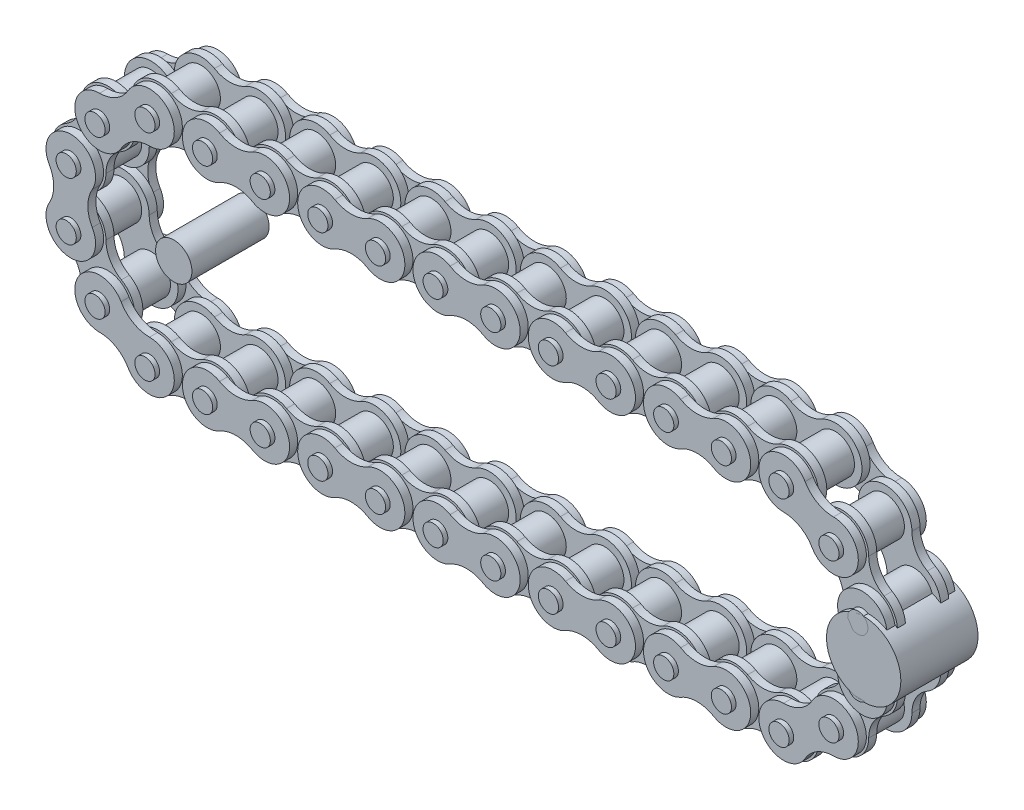
from build123d import *

# Parameters (mm, degrees)
EXTRUDE_1_DEPTH         = 8.500000462
EXTRUDE_1_DEPTH_BACK    = 8.500000462
SKETCH_1_R              = 2.224999946
EXTRUDE_1_2_DEPTH       = 8.500000462
EXTRUDE_1_2_DEPTH_BACK  = 8.500000462
EXTRUDE_1_3_DEPTH       = 8.500000462
EXTRUDE_1_3_DEPTH_BACK  = 8.500000462
EXTRUDE_1_4_DEPTH       = 8.500000462
EXTRUDE_1_4_DEPTH_BACK  = 8.500000462
EXTRUDE_1_5_DEPTH       = 8.500000462
EXTRUDE_1_5_DEPTH_BACK  = 8.500000462
EXTRUDE_1_6_DEPTH       = 8.500000462
EXTRUDE_1_6_DEPTH_BACK  = 8.500000462
EXTRUDE_1_7_DEPTH       = 8.500000462
EXTRUDE_1_7_DEPTH_BACK  = 8.500000462
EXTRUDE_1_8_DEPTH       = 8.500000462
EXTRUDE_1_8_DEPTH_BACK  = 8.500000462
EXTRUDE_1_9_DEPTH       = 8.500000462
EXTRUDE_1_9_DEPTH_BACK  = 8.500000462
EXTRUDE_1_10_DEPTH      = 8.500000462
EXTRUDE_1_10_DEPTH_BACK = 8.500000462
EXTRUDE_1_11_DEPTH      = 8.500000462
EXTRUDE_1_11_DEPTH_BACK = 8.500000462
EXTRUDE_1_12_DEPTH      = 8.500000462
EXTRUDE_1_12_DEPTH_BACK = 8.500000462
EXTRUDE_1_13_DEPTH      = 8.500000462
EXTRUDE_1_13_DEPTH_BACK = 8.500000462
EXTRUDE_1_14_DEPTH      = 8.500000462
EXTRUDE_1_14_DEPTH_BACK = 8.500000462
EXTRUDE_1_15_DEPTH      = 8.500000462
EXTRUDE_1_15_DEPTH_BACK = 8.500000462
EXTRUDE_1_16_DEPTH      = 8.500000462
EXTRUDE_1_16_DEPTH_BACK = 8.500000462
EXTRUDE_1_17_DEPTH      = 8.500000462
EXTRUDE_1_17_DEPTH_BACK = 8.500000462
EXTRUDE_1_18_DEPTH      = 8.500000462
EXTRUDE_1_18_DEPTH_BACK = 8.500000462
EXTRUDE_1_19_DEPTH      = 8.500000462
EXTRUDE_1_19_DEPTH_BACK = 8.500000462
EXTRUDE_1_20_DEPTH      = 8.500000462
EXTRUDE_1_20_DEPTH_BACK = 8.500000462
EXTRUDE_1_21_DEPTH      = 8.500000462
EXTRUDE_1_21_DEPTH_BACK = 8.500000462
EXTRUDE_1_22_DEPTH      = 8.500000462
EXTRUDE_1_22_DEPTH_BACK = 8.500000462
EXTRUDE_1_23_DEPTH      = 8.500000462
EXTRUDE_1_23_DEPTH_BACK = 8.500000462
EXTRUDE_1_24_DEPTH      = 8.500000462
EXTRUDE_1_24_DEPTH_BACK = 8.500000462
EXTRUDE_1_25_DEPTH      = 8.500000462
EXTRUDE_1_25_DEPTH_BACK = 8.500000462
EXTRUDE_1_26_DEPTH      = 8.500000462
EXTRUDE_1_26_DEPTH_BACK = 8.500000462
EXTRUDE_1_27_DEPTH      = 8.500000462
EXTRUDE_1_27_DEPTH_BACK = 8.500000462
EXTRUDE_1_28_DEPTH      = 8.500000462
EXTRUDE_1_28_DEPTH_BACK = 8.500000462
EXTRUDE_1_29_DEPTH      = 8.500000462
EXTRUDE_1_29_DEPTH_BACK = 8.500000462
EXTRUDE_1_30_DEPTH      = 8.500000462
EXTRUDE_1_30_DEPTH_BACK = 8.500000462
EXTRUDE_1_31_DEPTH      = 8.500000462
EXTRUDE_1_31_DEPTH_BACK = 8.500000462
EXTRUDE_1_32_DEPTH      = 8.500000462
EXTRUDE_1_32_DEPTH_BACK = 8.500000462
EXTRUDE_2_DEPTH         = 3.874999937
EXTRUDE_2_DEPTH_BACK    = 3.874999937
SKETCH_2_R              = 4.255000036
SKETCH_3_R              = 5.905000027
EXTRUDE_3_DEPTH         = 1.775000244
EXTRUDE_4_DEPTH         = 1.775000244
EXTRUDE_START           = 1.840000041
SKETCH_5_R              = 5.460000131
EXTRUDE_5_DEPTH         = 1.775000244
EXTRUDE_6_DEPTH         = 1.775000244
SKETCH_7_R              = 4.006025973
EXTRUDE_7_DEPTH         = 17.000000924
SKETCH_7_R_2            = 8.189187755
EXTRUDE_7_2_DEPTH       = 17.000000924


with BuildPart() as part:
    # 草图1 → 凸台-拉伸1 (new, two sides: drawn at the far end of the back side and taken through both)
    with BuildSketch(Plane.XY.offset(-EXTRUDE_1_DEPTH_BACK)):
        with Locations((-23.698522342, 6.349999923)):
            Circle(SKETCH_1_R)
    extrude(amount=EXTRUDE_1_DEPTH + EXTRUDE_1_DEPTH_BACK)



with BuildPart() as body_2:
    # 草图1 → Extrude 1 2 (new, two sides: drawn at the far end of the back side and taken through both)
    with BuildSketch(Plane.XY.offset(-EXTRUDE_1_2_DEPTH_BACK)):
        with Locations((-23.698522342, -6.349999923)):
            Circle(SKETCH_1_R)
    extrude(amount=EXTRUDE_1_2_DEPTH + EXTRUDE_1_2_DEPTH_BACK)


with BuildPart() as body_3:
    # 草图1 → Extrude 1 3 (new, two sides: drawn at the far end of the back side and taken through both)
    with BuildSketch(Plane.XY.offset(-EXTRUDE_1_3_DEPTH_BACK)):
        with Locations((150.698520807, 6.349999923)):
            Circle(SKETCH_1_R)
    extrude(amount=EXTRUDE_1_3_DEPTH + EXTRUDE_1_3_DEPTH_BACK)


with BuildPart() as body_4:
    # 草图1 → Extrude 1 4 (new, two sides: drawn at the far end of the back side and taken through both)
    with BuildSketch(Plane.XY.offset(-EXTRUDE_1_4_DEPTH_BACK)):
        with Locations((150.698520807, -6.349999923)):
            Circle(SKETCH_1_R)
    extrude(amount=EXTRUDE_1_4_DEPTH + EXTRUDE_1_4_DEPTH_BACK)


with BuildPart() as body_5:
    # 草图1 → Extrude 1 5 (new, two sides: drawn at the far end of the back side and taken through both)
    with BuildSketch(Plane.XY.offset(-EXTRUDE_1_5_DEPTH_BACK)):
        with Locations((-17.348522418, 17.348522418)):
            Circle(SKETCH_1_R)
    extrude(amount=EXTRUDE_1_5_DEPTH + EXTRUDE_1_5_DEPTH_BACK)


with BuildPart() as body_6:
    # 草图1 → Extrude 1 6 (new, two sides: drawn at the far end of the back side and taken through both)
    with BuildSketch(Plane.XY.offset(-EXTRUDE_1_6_DEPTH_BACK)):
        with Locations((-17.348522418, -17.348522418)):
            Circle(SKETCH_1_R)
    extrude(amount=EXTRUDE_1_6_DEPTH + EXTRUDE_1_6_DEPTH_BACK)


with BuildPart() as body_7:
    # 草图1 → Extrude 1 7 (new, two sides: drawn at the far end of the back side and taken through both)
    with BuildSketch(Plane.XY.offset(-EXTRUDE_1_7_DEPTH_BACK)):
        with Locations((-6.349999923, 23.698522342)):
            Circle(SKETCH_1_R)
    extrude(amount=EXTRUDE_1_7_DEPTH + EXTRUDE_1_7_DEPTH_BACK)


with BuildPart() as body_8:
    # 草图1 → Extrude 1 8 (new, two sides: drawn at the far end of the back side and taken through both)
    with BuildSketch(Plane.XY.offset(-EXTRUDE_1_8_DEPTH_BACK)):
        with Locations((-6.349999923, -23.698522342)):
            Circle(SKETCH_1_R)
    extrude(amount=EXTRUDE_1_8_DEPTH + EXTRUDE_1_8_DEPTH_BACK)


with BuildPart() as body_9:
    # 草图1 → Extrude 1 9 (new, two sides: drawn at the far end of the back side and taken through both)
    with BuildSketch(Plane.XY.offset(-EXTRUDE_1_9_DEPTH_BACK)):
        with Locations((144.348520884, 17.348522418)):
            Circle(SKETCH_1_R)
    extrude(amount=EXTRUDE_1_9_DEPTH + EXTRUDE_1_9_DEPTH_BACK)


with BuildPart() as body_10:
    # 草图1 → Extrude 1 10 (new, two sides: drawn at the far end of the back side and taken through both)
    with BuildSketch(Plane.XY.offset(-EXTRUDE_1_10_DEPTH_BACK)):
        with Locations((144.348520884, -17.348522418)):
            Circle(SKETCH_1_R)
    extrude(amount=EXTRUDE_1_10_DEPTH + EXTRUDE_1_10_DEPTH_BACK)


with BuildPart() as body_11:
    # 草图1 → Extrude 1 11 (new, two sides: drawn at the far end of the back side and taken through both)
    with BuildSketch(Plane.XY.offset(-EXTRUDE_1_11_DEPTH_BACK)):
        with Locations((133.349998388, 23.698522342)):
            Circle(SKETCH_1_R)
    extrude(amount=EXTRUDE_1_11_DEPTH + EXTRUDE_1_11_DEPTH_BACK)


with BuildPart() as body_12:
    # 草图1 → Extrude 1 12 (new, two sides: drawn at the far end of the back side and taken through both)
    with BuildSketch(Plane.XY.offset(-EXTRUDE_1_12_DEPTH_BACK)):
        with Locations((133.349998388, -23.698522342)):
            Circle(SKETCH_1_R)
    extrude(amount=EXTRUDE_1_12_DEPTH + EXTRUDE_1_12_DEPTH_BACK)


with BuildPart() as body_13:
    # 草图1 → Extrude 1 13 (new, two sides: drawn at the far end of the back side and taken through both)
    with BuildSketch(Plane.XY.offset(-EXTRUDE_1_13_DEPTH_BACK)):
        with Locations((6.349999923, 23.698522342)):
            Circle(SKETCH_1_R)
    extrude(amount=EXTRUDE_1_13_DEPTH + EXTRUDE_1_13_DEPTH_BACK)


with BuildPart() as body_14:
    # 草图1 → Extrude 1 14 (new, two sides: drawn at the far end of the back side and taken through both)
    with BuildSketch(Plane.XY.offset(-EXTRUDE_1_14_DEPTH_BACK)):
        with Locations((6.349999923, -23.698522342)):
            Circle(SKETCH_1_R)
    extrude(amount=EXTRUDE_1_14_DEPTH + EXTRUDE_1_14_DEPTH_BACK)


with BuildPart() as body_15:
    # 草图1 → Extrude 1 15 (new, two sides: drawn at the far end of the back side and taken through both)
    with BuildSketch(Plane.XY.offset(-EXTRUDE_1_15_DEPTH_BACK)):
        with Locations((19.04999977, 23.698522342)):
            Circle(SKETCH_1_R)
    extrude(amount=EXTRUDE_1_15_DEPTH + EXTRUDE_1_15_DEPTH_BACK)


with BuildPart() as body_16:
    # 草图1 → Extrude 1 16 (new, two sides: drawn at the far end of the back side and taken through both)
    with BuildSketch(Plane.XY.offset(-EXTRUDE_1_16_DEPTH_BACK)):
        with Locations((19.04999977, -23.698522342)):
            Circle(SKETCH_1_R)
    extrude(amount=EXTRUDE_1_16_DEPTH + EXTRUDE_1_16_DEPTH_BACK)


with BuildPart() as body_17:
    # 草图1 → Extrude 1 17 (new, two sides: drawn at the far end of the back side and taken through both)
    with BuildSketch(Plane.XY.offset(-EXTRUDE_1_17_DEPTH_BACK)):
        with Locations((31.749999616, 23.698522342)):
            Circle(SKETCH_1_R)
    extrude(amount=EXTRUDE_1_17_DEPTH + EXTRUDE_1_17_DEPTH_BACK)


with BuildPart() as body_18:
    # 草图1 → Extrude 1 18 (new, two sides: drawn at the far end of the back side and taken through both)
    with BuildSketch(Plane.XY.offset(-EXTRUDE_1_18_DEPTH_BACK)):
        with Locations((31.749999616, -23.698522342)):
            Circle(SKETCH_1_R)
    extrude(amount=EXTRUDE_1_18_DEPTH + EXTRUDE_1_18_DEPTH_BACK)


with BuildPart() as body_19:
    # 草图1 → Extrude 1 19 (new, two sides: drawn at the far end of the back side and taken through both)
    with BuildSketch(Plane.XY.offset(-EXTRUDE_1_19_DEPTH_BACK)):
        with Locations((44.449999463, 23.698522342)):
            Circle(SKETCH_1_R)
    extrude(amount=EXTRUDE_1_19_DEPTH + EXTRUDE_1_19_DEPTH_BACK)


with BuildPart() as body_20:
    # 草图1 → Extrude 1 20 (new, two sides: drawn at the far end of the back side and taken through both)
    with BuildSketch(Plane.XY.offset(-EXTRUDE_1_20_DEPTH_BACK)):
        with Locations((44.449999463, -23.698522342)):
            Circle(SKETCH_1_R)
    extrude(amount=EXTRUDE_1_20_DEPTH + EXTRUDE_1_20_DEPTH_BACK)


with BuildPart() as body_21:
    # 草图1 → Extrude 1 21 (new, two sides: drawn at the far end of the back side and taken through both)
    with BuildSketch(Plane.XY.offset(-EXTRUDE_1_21_DEPTH_BACK)):
        with Locations((57.149999309, 23.698522342)):
            Circle(SKETCH_1_R)
    extrude(amount=EXTRUDE_1_21_DEPTH + EXTRUDE_1_21_DEPTH_BACK)


with BuildPart() as body_22:
    # 草图1 → Extrude 1 22 (new, two sides: drawn at the far end of the back side and taken through both)
    with BuildSketch(Plane.XY.offset(-EXTRUDE_1_22_DEPTH_BACK)):
        with Locations((57.149999309, -23.698522342)):
            Circle(SKETCH_1_R)
    extrude(amount=EXTRUDE_1_22_DEPTH + EXTRUDE_1_22_DEPTH_BACK)


with BuildPart() as body_23:
    # 草图1 → Extrude 1 23 (new, two sides: drawn at the far end of the back side and taken through both)
    with BuildSketch(Plane.XY.offset(-EXTRUDE_1_23_DEPTH_BACK)):
        with Locations((69.849999156, 23.698522342)):
            Circle(SKETCH_1_R)
    extrude(amount=EXTRUDE_1_23_DEPTH + EXTRUDE_1_23_DEPTH_BACK)


with BuildPart() as body_24:
    # 草图1 → Extrude 1 24 (new, two sides: drawn at the far end of the back side and taken through both)
    with BuildSketch(Plane.XY.offset(-EXTRUDE_1_24_DEPTH_BACK)):
        with Locations((69.849999156, -23.698522342)):
            Circle(SKETCH_1_R)
    extrude(amount=EXTRUDE_1_24_DEPTH + EXTRUDE_1_24_DEPTH_BACK)


with BuildPart() as body_25:
    # 草图1 → Extrude 1 25 (new, two sides: drawn at the far end of the back side and taken through both)
    with BuildSketch(Plane.XY.offset(-EXTRUDE_1_25_DEPTH_BACK)):
        with Locations((82.549999002, 23.698522342)):
            Circle(SKETCH_1_R)
    extrude(amount=EXTRUDE_1_25_DEPTH + EXTRUDE_1_25_DEPTH_BACK)


with BuildPart() as body_26:
    # 草图1 → Extrude 1 26 (new, two sides: drawn at the far end of the back side and taken through both)
    with BuildSketch(Plane.XY.offset(-EXTRUDE_1_26_DEPTH_BACK)):
        with Locations((82.549999002, -23.698522342)):
            Circle(SKETCH_1_R)
    extrude(amount=EXTRUDE_1_26_DEPTH + EXTRUDE_1_26_DEPTH_BACK)


with BuildPart() as body_27:
    # 草图1 → Extrude 1 27 (new, two sides: drawn at the far end of the back side and taken through both)
    with BuildSketch(Plane.XY.offset(-EXTRUDE_1_27_DEPTH_BACK)):
        with Locations((95.249998849, 23.698522342)):
            Circle(SKETCH_1_R)
    extrude(amount=EXTRUDE_1_27_DEPTH + EXTRUDE_1_27_DEPTH_BACK)


with BuildPart() as body_28:
    # 草图1 → Extrude 1 28 (new, two sides: drawn at the far end of the back side and taken through both)
    with BuildSketch(Plane.XY.offset(-EXTRUDE_1_28_DEPTH_BACK)):
        with Locations((95.249998849, -23.698522342)):
            Circle(SKETCH_1_R)
    extrude(amount=EXTRUDE_1_28_DEPTH + EXTRUDE_1_28_DEPTH_BACK)


with BuildPart() as body_29:
    # 草图1 → Extrude 1 29 (new, two sides: drawn at the far end of the back side and taken through both)
    with BuildSketch(Plane.XY.offset(-EXTRUDE_1_29_DEPTH_BACK)):
        with Locations((107.949998695, 23.698522342)):
            Circle(SKETCH_1_R)
    extrude(amount=EXTRUDE_1_29_DEPTH + EXTRUDE_1_29_DEPTH_BACK)


with BuildPart() as body_30:
    # 草图1 → Extrude 1 30 (new, two sides: drawn at the far end of the back side and taken through both)
    with BuildSketch(Plane.XY.offset(-EXTRUDE_1_30_DEPTH_BACK)):
        with Locations((107.949998695, -23.698522342)):
            Circle(SKETCH_1_R)
    extrude(amount=EXTRUDE_1_30_DEPTH + EXTRUDE_1_30_DEPTH_BACK)


with BuildPart() as body_31:
    # 草图1 → Extrude 1 31 (new, two sides: drawn at the far end of the back side and taken through both)
    with BuildSketch(Plane.XY.offset(-EXTRUDE_1_31_DEPTH_BACK)):
        with Locations((120.649998542, 23.698522342)):
            Circle(SKETCH_1_R)
    extrude(amount=EXTRUDE_1_31_DEPTH + EXTRUDE_1_31_DEPTH_BACK)


with BuildPart() as body_32:
    # 草图1 → Extrude 1 32 (new, two sides: drawn at the far end of the back side and taken through both)
    with BuildSketch(Plane.XY.offset(-EXTRUDE_1_32_DEPTH_BACK)):
        with Locations((120.649998542, -23.698522342)):
            Circle(SKETCH_1_R)
    extrude(amount=EXTRUDE_1_32_DEPTH + EXTRUDE_1_32_DEPTH_BACK)


with BuildPart() as part_1:
    add(part.part)

    add(body_2.part)  # 凸台-拉伸2 merges body 2

    add(body_3.part)  # 凸台-拉伸2 merges body 3

    add(body_4.part)  # 凸台-拉伸2 merges body 4

    add(body_5.part)  # 凸台-拉伸2 merges body 5

    add(body_6.part)  # 凸台-拉伸2 merges body 6

    add(body_7.part)  # 凸台-拉伸2 merges body 7

    add(body_8.part)  # 凸台-拉伸2 merges body 8

    add(body_9.part)  # 凸台-拉伸2 merges body 9

    add(body_10.part)  # 凸台-拉伸2 merges body 10

    add(body_11.part)  # 凸台-拉伸2 merges body 11

    add(body_12.part)  # 凸台-拉伸2 merges body 12

    add(body_13.part)  # 凸台-拉伸2 merges body 13

    add(body_14.part)  # 凸台-拉伸2 merges body 14

    add(body_15.part)  # 凸台-拉伸2 merges body 15

    add(body_16.part)  # 凸台-拉伸2 merges body 16

    add(body_17.part)  # 凸台-拉伸2 merges body 17

    add(body_18.part)  # 凸台-拉伸2 merges body 18

    add(body_19.part)  # 凸台-拉伸2 merges body 19

    add(body_20.part)  # 凸台-拉伸2 merges body 20

    add(body_21.part)  # 凸台-拉伸2 merges body 21

    add(body_22.part)  # 凸台-拉伸2 merges body 22

    add(body_23.part)  # 凸台-拉伸2 merges body 23

    add(body_24.part)  # 凸台-拉伸2 merges body 24

    add(body_25.part)  # 凸台-拉伸2 merges body 25

    add(body_26.part)  # 凸台-拉伸2 merges body 26

    add(body_27.part)  # 凸台-拉伸2 merges body 27

    add(body_28.part)  # 凸台-拉伸2 merges body 28

    add(body_29.part)  # 凸台-拉伸2 merges body 29

    add(body_30.part)  # 凸台-拉伸2 merges body 30

    add(body_31.part)  # 凸台-拉伸2 merges body 31

    add(body_32.part)  # 凸台-拉伸2 merges body 32
    # 草图2 → 凸台-拉伸2 (add, two sides: drawn at the far end of the back side and taken through both)
    with BuildSketch(Plane.XY.offset(-EXTRUDE_2_DEPTH_BACK)):
        with Locations((-23.698522342, 6.349999923)):
            Circle(SKETCH_2_R)
        with Locations((-23.698522342, -6.349999923)):
            Circle(SKETCH_2_R)
        with Locations((150.698520807, 6.349999923)):
            Circle(SKETCH_2_R)
        with Locations((150.698520807, -6.349999923)):
            Circle(SKETCH_2_R)
        with Locations((-17.348522418, 17.348522418)):
            Circle(SKETCH_2_R)
        with Locations((-17.348522418, -17.348522418)):
            Circle(SKETCH_2_R)
        with Locations((-6.349999923, 23.698522342)):
            Circle(SKETCH_2_R)
        with Locations((-6.349999923, -23.698522342)):
            Circle(SKETCH_2_R)
        with Locations((144.348520884, 17.348522418)):
            Circle(SKETCH_2_R)
        with Locations((144.348520884, -17.348522418)):
            Circle(SKETCH_2_R)
        with Locations((133.349998388, 23.698522342)):
            Circle(SKETCH_2_R)
        with Locations((133.349998388, -23.698522342)):
            Circle(SKETCH_2_R)
        with Locations((6.349999923, 23.698522342)):
            Circle(SKETCH_2_R)
        with Locations((6.349999923, -23.698522342)):
            Circle(SKETCH_2_R)
        with Locations((19.04999977, 23.698522342)):
            Circle(SKETCH_2_R)
        with Locations((19.04999977, -23.698522342)):
            Circle(SKETCH_2_R)
        with Locations((31.749999616, 23.698522342)):
            Circle(SKETCH_2_R)
        with Locations((31.749999616, -23.698522342)):
            Circle(SKETCH_2_R)
        with Locations((44.449999463, 23.698522342)):
            Circle(SKETCH_2_R)
        with Locations((44.449999463, -23.698522342)):
            Circle(SKETCH_2_R)
        with Locations((57.149999309, 23.698522342)):
            Circle(SKETCH_2_R)
        with Locations((57.149999309, -23.698522342)):
            Circle(SKETCH_2_R)
        with Locations((69.849999156, 23.698522342)):
            Circle(SKETCH_2_R)
        with Locations((69.849999156, -23.698522342)):
            Circle(SKETCH_2_R)
        with Locations((82.549999002, 23.698522342)):
            Circle(SKETCH_2_R)
        with Locations((82.549999002, -23.698522342)):
            Circle(SKETCH_2_R)
        with Locations((95.249998849, 23.698522342)):
            Circle(SKETCH_2_R)
        with Locations((95.249998849, -23.698522342)):
            Circle(SKETCH_2_R)
        with Locations((107.949998695, 23.698522342)):
            Circle(SKETCH_2_R)
        with Locations((107.949998695, -23.698522342)):
            Circle(SKETCH_2_R)
        with Locations((120.649998542, 23.698522342)):
            Circle(SKETCH_2_R)
        with Locations((120.649998542, -23.698522342)):
            Circle(SKETCH_2_R)
    extrude(amount=EXTRUDE_2_DEPTH + EXTRUDE_2_DEPTH_BACK)

    # 草图3 → 凸台-拉伸3 (add)
    with BuildSketch(Plane.XY.offset(3.874999937)):
        with Locations(Location((-23.698522342, 6.349999923, 0), (0, 0, 180))):
            Circle(SKETCH_3_R)
        with Locations(Location((-23.698522342, -6.349999923, 0), (0, 0, 180))):
            Circle(SKETCH_3_R)
        with Locations(Location((150.698520807, 6.349999923, 0), (0, 0, 180))):
            Circle(SKETCH_3_R)
        with Locations(Location((150.698520807, -6.349999923, 0), (0, 0, 180))):
            Circle(SKETCH_3_R)
        with Locations(Location((-17.348522418, 17.348522418, 0), (0, 0, 180))):
            Circle(SKETCH_3_R)
        with Locations(Location((-17.348522418, -17.348522418, 0), (0, 0, 180))):
            Circle(SKETCH_3_R)
        with Locations(Location((-6.349999923, 23.698522342, 0), (0, 0, 180))):
            Circle(SKETCH_3_R)
        with Locations(Location((-6.349999923, -23.698522342, 0), (0, 0, 180))):
            Circle(SKETCH_3_R)
        with Locations(Location((144.348520884, 17.348522418, 0), (0, 0, 180))):
            Circle(SKETCH_3_R)
        with Locations(Location((144.348520884, -17.348522418, 0), (0, 0, 180))):
            Circle(SKETCH_3_R)
        with Locations(Location((133.349998388, 23.698522342, 0), (0, 0, 180))):
            Circle(SKETCH_3_R)
        with Locations(Location((133.349998388, -23.698522342, 0), (0, 0, 180))):
            Circle(SKETCH_3_R)
        with Locations(Location((6.349999923, 23.698522342, 0), (0, 0, 180))):
            Circle(SKETCH_3_R)
        with Locations(Location((6.349999923, -23.698522342, 0), (0, 0, 180))):
            Circle(SKETCH_3_R)
        with Locations(Location((19.04999977, 23.698522342, 0), (0, 0, 180))):
            Circle(SKETCH_3_R)
        with Locations(Location((19.04999977, -23.698522342, 0), (0, 0, 180))):
            Circle(SKETCH_3_R)
        with Locations(Location((31.749999616, 23.698522342, 0), (0, 0, 180))):
            Circle(SKETCH_3_R)
        with Locations(Location((31.749999616, -23.698522342, 0), (0, 0, 180))):
            Circle(SKETCH_3_R)
        with Locations(Location((44.449999463, 23.698522342, 0), (0, 0, 180))):
            Circle(SKETCH_3_R)
        with Locations(Location((44.449999463, -23.698522342, 0), (0, 0, 180))):
            Circle(SKETCH_3_R)
        with Locations(Location((57.149999309, 23.698522342, 0), (0, 0, 180))):
            Circle(SKETCH_3_R)
        with Locations(Location((57.149999309, -23.698522342, 0), (0, 0, 180))):
            Circle(SKETCH_3_R)
        with Locations(Location((69.849999156, 23.698522342, 0), (0, 0, 180))):
            Circle(SKETCH_3_R)
        with Locations(Location((69.849999156, -23.698522342, 0), (0, 0, 180))):
            Circle(SKETCH_3_R)
        with Locations(Location((82.549999002, 23.698522342, 0), (0, 0, 180))):
            Circle(SKETCH_3_R)
        with Locations(Location((82.549999002, -23.698522342, 0), (0, 0, 180))):
            Circle(SKETCH_3_R)
        with Locations(Location((95.249998849, 23.698522342, 0), (0, 0, 180))):
            Circle(SKETCH_3_R)
        with Locations(Location((95.249998849, -23.698522342, 0), (0, 0, 180))):
            Circle(SKETCH_3_R)
        with Locations(Location((107.949998695, 23.698522342, 0), (0, 0, 180))):
            Circle(SKETCH_3_R)
        with Locations(Location((107.949998695, -23.698522342, 0), (0, 0, 180))):
            Circle(SKETCH_3_R)
        with Locations(Location((120.649998542, 23.698522342, 0), (0, 0, 180))):
            Circle(SKETCH_3_R)
        with Locations(Location((120.649998542, -23.698522342, 0), (0, 0, 180))):
            Circle(SKETCH_3_R)
    extrude_3 = extrude(amount=EXTRUDE_3_DEPTH)

    # 草图4 → 凸台-拉伸4 (add)
    with BuildSketch(Plane.XY.offset(3.874999937)):
        with BuildLine():
            Line((-26.651022364, 11.463879961), (-17.793522323, 6.349999928))
            ThreePointArc((-17.793522323, 6.349999928), (-16.883164966, 9.747499838), (-14.396022414, 12.234642391))
            Line((-14.396022414, 12.234642391), (-23.253522455, 17.348522424))
            ThreePointArc((-23.253522455, 17.348522424), (-24.163879812, 13.951022514), (-26.651022364, 11.463879961))
        make_face()
        with BuildLine():
            Line((-26.651022364, -11.463879961), (-17.793522323, -6.349999928))
            ThreePointArc((-17.793522323, -6.349999928), (-16.883164966, -9.747499838), (-14.396022414, -12.234642391))
            Line((-14.396022414, -12.234642391), (-23.253522455, -17.348522424))
            ThreePointArc((-23.253522455, -17.348522424), (-24.163879812, -13.951022514), (-26.651022364, -11.463879961))
        make_face()
        with BuildLine():
            Line((153.65102082, 11.463879956), (144.79352078, 6.349999923))
            ThreePointArc((144.79352078, 6.349999923), (143.883163423, 9.747499833), (141.39602087, 12.234642385))
            Line((141.39602087, 12.234642385), (150.253520911, 17.348522418))
            ThreePointArc((150.253520911, 17.348522418), (151.163878268, 13.951022509), (153.65102082, 11.463879956))
        make_face()
        with BuildLine():
            Line((153.65102082, -11.463879956), (144.79352078, -6.349999923))
            ThreePointArc((144.79352078, -6.349999923), (143.883163423, -9.747499833), (141.39602087, -12.234642385))
            Line((141.39602087, -12.234642385), (150.253520911, -17.348522418))
            ThreePointArc((150.253520911, -17.348522418), (151.163878268, -13.951022509), (153.65102082, -11.463879956))
        make_face()
        with BuildLine():
            Line((-3.39749991, 28.812402375), (-3.39749991, 18.584642309))
            ThreePointArc((-3.39749991, 18.584642309), (0, 19.494999666), (3.39749991, 18.584642309))
            Line((3.39749991, 18.584642309), (3.39749991, 28.812402375))
            ThreePointArc((3.39749991, 28.812402375), (0, 27.902045018), (-3.39749991, 28.812402375))
        make_face()
        with BuildLine():
            Line((-3.39749991, -28.812402375), (-3.39749991, -18.584642309))
            ThreePointArc((-3.39749991, -18.584642309), (0, -19.494999666), (3.39749991, -18.584642309))
            Line((3.39749991, -18.584642309), (3.39749991, -28.812402375))
            ThreePointArc((3.39749991, -28.812402375), (0, -27.902045018), (-3.39749991, -28.812402375))
        make_face()
        with BuildLine():
            Line((22.002499783, 28.812402375), (22.002499783, 18.584642309))
            ThreePointArc((22.002499783, 18.584642309), (25.399999693, 19.494999666), (28.797499603, 18.584642309))
            Line((28.797499603, 18.584642309), (28.797499603, 28.812402375))
            ThreePointArc((28.797499603, 28.812402375), (25.399999693, 27.902045018), (22.002499783, 28.812402375))
        make_face()
        with BuildLine():
            Line((22.002499783, -28.812402375), (22.002499783, -18.584642309))
            ThreePointArc((22.002499783, -18.584642309), (25.399999693, -19.494999666), (28.797499603, -18.584642309))
            Line((28.797499603, -18.584642309), (28.797499603, -28.812402375))
            ThreePointArc((28.797499603, -28.812402375), (25.399999693, -27.902045018), (22.002499783, -28.812402375))
        make_face()
        with BuildLine():
            Line((47.402499476, 28.812402375), (47.402499476, 18.584642309))
            ThreePointArc((47.402499476, 18.584642309), (50.799999386, 19.494999666), (54.197499296, 18.584642309))
            Line((54.197499296, 18.584642309), (54.197499296, 28.812402375))
            ThreePointArc((54.197499296, 28.812402375), (50.799999386, 27.902045018), (47.402499476, 28.812402375))
        make_face()
        with BuildLine():
            Line((47.402499476, -28.812402375), (47.402499476, -18.584642309))
            ThreePointArc((47.402499476, -18.584642309), (50.799999386, -19.494999666), (54.197499296, -18.584642309))
            Line((54.197499296, -18.584642309), (54.197499296, -28.812402375))
            ThreePointArc((54.197499296, -28.812402375), (50.799999386, -27.902045018), (47.402499476, -28.812402375))
        make_face()
        with BuildLine():
            Line((72.802499169, 28.812402375), (72.802499169, 18.584642309))
            ThreePointArc((72.802499169, 18.584642309), (76.199999079, 19.494999666), (79.597498989, 18.584642309))
            Line((79.597498989, 18.584642309), (79.597498989, 28.812402375))
            ThreePointArc((79.597498989, 28.812402375), (76.199999079, 27.902045018), (72.802499169, 28.812402375))
        make_face()
        with BuildLine():
            Line((72.802499169, -28.812402375), (72.802499169, -18.584642309))
            ThreePointArc((72.802499169, -18.584642309), (76.199999079, -19.494999666), (79.597498989, -18.584642309))
            Line((79.597498989, -18.584642309), (79.597498989, -28.812402375))
            ThreePointArc((79.597498989, -28.812402375), (76.199999079, -27.902045018), (72.802499169, -28.812402375))
        make_face()
        with BuildLine():
            Line((98.202498863, 28.812402375), (98.202498863, 18.584642309))
            ThreePointArc((98.202498863, 18.584642309), (101.599998772, 19.494999666), (104.997498682, 18.584642309))
            Line((104.997498682, 18.584642309), (104.997498682, 28.812402375))
            ThreePointArc((104.997498682, 28.812402375), (101.599998772, 27.902045018), (98.202498863, 28.812402375))
        make_face()
        with BuildLine():
            Line((98.202498863, -28.812402375), (98.202498863, -18.584642309))
            ThreePointArc((98.202498863, -18.584642309), (101.599998772, -19.494999666), (104.997498682, -18.584642309))
            Line((104.997498682, -18.584642309), (104.997498682, -28.812402375))
            ThreePointArc((104.997498682, -28.812402375), (101.599998772, -27.902045018), (98.202498863, -28.812402375))
        make_face()
        with BuildLine():
            Line((123.602498556, 28.812402375), (123.602498556, 18.584642309))
            ThreePointArc((123.602498556, 18.584642309), (126.999998465, 19.494999666), (130.397498375, 18.584642309))
            Line((130.397498375, 18.584642309), (130.397498375, 28.812402375))
            ThreePointArc((130.397498375, 28.812402375), (126.999998465, 27.902045018), (123.602498556, 28.812402375))
        make_face()
        with BuildLine():
            Line((123.602498556, -28.812402375), (123.602498556, -18.584642309))
            ThreePointArc((123.602498556, -18.584642309), (126.999998465, -19.494999666), (130.397498375, -18.584642309))
            Line((130.397498375, -18.584642309), (130.397498375, -28.812402375))
            ThreePointArc((130.397498375, -28.812402375), (126.999998465, -27.902045018), (123.602498556, -28.812402375))
        make_face()
    extrude_4 = extrude(amount=EXTRUDE_4_DEPTH)

    # 草图5 → 凸台-拉伸5 (add)
    with BuildSketch(Plane.XY.offset(3.874999937).offset(EXTRUDE_START)):
        with Locations(Location((-23.698522342, 6.349999923, 0), (0, 0, 180))):
            Circle(SKETCH_5_R)
        with Locations(Location((-23.698522342, -6.349999923, 0), (0, 0, 180))):
            Circle(SKETCH_5_R)
        with Locations(Location((150.698520807, 6.349999923, 0), (0, 0, 180))):
            Circle(SKETCH_5_R)
        with Locations(Location((150.698520807, -6.349999923, 0), (0, 0, 180))):
            Circle(SKETCH_5_R)
        with Locations(Location((-17.348522418, 17.348522418, 0), (0, 0, 180))):
            Circle(SKETCH_5_R)
        with Locations(Location((-17.348522418, -17.348522418, 0), (0, 0, 180))):
            Circle(SKETCH_5_R)
        with Locations(Location((-6.349999923, 23.698522342, 0), (0, 0, 180))):
            Circle(SKETCH_5_R)
        with Locations(Location((-6.349999923, -23.698522342, 0), (0, 0, 180))):
            Circle(SKETCH_5_R)
        with Locations(Location((144.348520884, 17.348522418, 0), (0, 0, 180))):
            Circle(SKETCH_5_R)
        with Locations(Location((144.348520884, -17.348522418, 0), (0, 0, 180))):
            Circle(SKETCH_5_R)
        with Locations(Location((133.349998388, 23.698522342, 0), (0, 0, 180))):
            Circle(SKETCH_5_R)
        with Locations(Location((133.349998388, -23.698522342, 0), (0, 0, 180))):
            Circle(SKETCH_5_R)
        with Locations(Location((6.349999923, 23.698522342, 0), (0, 0, 180))):
            Circle(SKETCH_5_R)
        with Locations(Location((6.349999923, -23.698522342, 0), (0, 0, 180))):
            Circle(SKETCH_5_R)
        with Locations(Location((19.04999977, 23.698522342, 0), (0, 0, 180))):
            Circle(SKETCH_5_R)
        with Locations(Location((19.04999977, -23.698522342, 0), (0, 0, 180))):
            Circle(SKETCH_5_R)
        with Locations(Location((31.749999616, 23.698522342, 0), (0, 0, 180))):
            Circle(SKETCH_5_R)
        with Locations(Location((31.749999616, -23.698522342, 0), (0, 0, 180))):
            Circle(SKETCH_5_R)
        with Locations(Location((44.449999463, 23.698522342, 0), (0, 0, 180))):
            Circle(SKETCH_5_R)
        with Locations(Location((44.449999463, -23.698522342, 0), (0, 0, 180))):
            Circle(SKETCH_5_R)
        with Locations(Location((57.149999309, 23.698522342, 0), (0, 0, 180))):
            Circle(SKETCH_5_R)
        with Locations(Location((57.149999309, -23.698522342, 0), (0, 0, 180))):
            Circle(SKETCH_5_R)
        with Locations(Location((69.849999156, 23.698522342, 0), (0, 0, 180))):
            Circle(SKETCH_5_R)
        with Locations(Location((69.849999156, -23.698522342, 0), (0, 0, 180))):
            Circle(SKETCH_5_R)
        with Locations(Location((82.549999002, 23.698522342, 0), (0, 0, 180))):
            Circle(SKETCH_5_R)
        with Locations(Location((82.549999002, -23.698522342, 0), (0, 0, 180))):
            Circle(SKETCH_5_R)
        with Locations(Location((95.249998849, 23.698522342, 0), (0, 0, 180))):
            Circle(SKETCH_5_R)
        with Locations(Location((95.249998849, -23.698522342, 0), (0, 0, 180))):
            Circle(SKETCH_5_R)
        with Locations(Location((107.949998695, 23.698522342, 0), (0, 0, 180))):
            Circle(SKETCH_5_R)
        with Locations(Location((107.949998695, -23.698522342, 0), (0, 0, 180))):
            Circle(SKETCH_5_R)
        with Locations(Location((120.649998542, 23.698522342, 0), (0, 0, 180))):
            Circle(SKETCH_5_R)
        with Locations(Location((120.649998542, -23.698522342, 0), (0, 0, 180))):
            Circle(SKETCH_5_R)
    extrude_5 = extrude(amount=EXTRUDE_5_DEPTH)

    # 草图6 → 凸台-拉伸6 (add)
    with BuildSketch(Plane.XY.offset(3.874999937).offset(EXTRUDE_START)):
        with BuildLine():
            Line((-28.42702117, 3.619999858), (-18.970023534, 3.619999858))
            ThreePointArc((-18.970023534, 3.619999858), (-19.939999572, 0), (-18.970023534, -3.619999858))
            Line((-18.970023534, -3.619999858), (-28.42702117, -3.619999858))
            ThreePointArc((-28.42702117, -3.619999858), (-27.457045132, 0), (-28.42702117, 3.619999858))
        make_face()
        with BuildLine():
            Line((155.427019625, 3.619999858), (145.970021988, 3.619999858))
            ThreePointArc((145.970021988, 3.619999858), (146.939998027, 0), (145.970021988, -3.619999858))
            Line((145.970021988, -3.619999858), (155.427019625, -3.619999858))
            ThreePointArc((155.427019625, -3.619999858), (154.457043587, 0), (155.427019625, 3.619999858))
        make_face()
        with BuildLine():
            Line((-17.348522424, 22.808522559), (-12.620023605, 14.618522362))
            ThreePointArc((-12.620023605, 14.618522362), (-9.969999786, 17.268546181), (-6.349999928, 18.238522219))
            Line((-6.349999928, 18.238522219), (-11.078498747, 26.428522416))
            ThreePointArc((-11.078498747, 26.428522416), (-13.728522566, 23.778498597), (-17.348522424, 22.808522559))
        make_face()
        with BuildLine():
            Line((-17.348522424, -22.808522559), (-12.620023605, -14.618522362))
            ThreePointArc((-12.620023605, -14.618522362), (-9.969999786, -17.268546181), (-6.349999928, -18.238522219))
            Line((-6.349999928, -18.238522219), (-11.078498747, -26.428522416))
            ThreePointArc((-11.078498747, -26.428522416), (-13.728522566, -23.778498597), (-17.348522424, -22.808522559))
        make_face()
        with BuildLine():
            Line((144.348520884, 22.80852255), (139.620022065, 14.618522353))
            ThreePointArc((139.620022065, 14.618522353), (136.969998246, 17.268546172), (133.349998388, 18.23852221))
            Line((133.349998388, 18.23852221), (138.078497207, 26.428522407))
            ThreePointArc((138.078497207, 26.428522407), (140.728521026, 23.778498588), (144.348520884, 22.80852255))
        make_face()
        with BuildLine():
            Line((144.348520884, -22.80852255), (139.620022065, -14.618522353))
            ThreePointArc((139.620022065, -14.618522353), (136.969998246, -17.268546172), (133.349998388, -18.23852221))
            Line((133.349998388, -18.23852221), (138.078497207, -26.428522407))
            ThreePointArc((138.078497207, -26.428522407), (140.728521026, -23.778498588), (144.348520884, -22.80852255))
        make_face()
        with BuildLine():
            Line((9.079999989, 28.42702116), (9.079999989, 18.970023523))
            ThreePointArc((9.079999989, 18.970023523), (12.699999847, 19.939999562), (16.319999704, 18.970023523))
            Line((16.319999704, 18.970023523), (16.319999704, 28.42702116))
            ThreePointArc((16.319999704, 28.42702116), (12.699999847, 27.457045122), (9.079999989, 28.42702116))
        make_face()
        with BuildLine():
            Line((9.079999989, -28.42702116), (9.079999989, -18.970023523))
            ThreePointArc((9.079999989, -18.970023523), (12.699999847, -19.939999562), (16.319999704, -18.970023523))
            Line((16.319999704, -18.970023523), (16.319999704, -28.42702116))
            ThreePointArc((16.319999704, -28.42702116), (12.699999847, -27.457045122), (9.079999989, -28.42702116))
        make_face()
        with BuildLine():
            Line((34.479999682, 28.42702116), (34.479999682, 18.970023523))
            ThreePointArc((34.479999682, 18.970023523), (38.09999954, 19.939999562), (41.719999397, 18.970023523))
            Line((41.719999397, 18.970023523), (41.719999397, 28.42702116))
            ThreePointArc((41.719999397, 28.42702116), (38.09999954, 27.457045122), (34.479999682, 28.42702116))
        make_face()
        with BuildLine():
            Line((34.479999682, -28.42702116), (34.479999682, -18.970023523))
            ThreePointArc((34.479999682, -18.970023523), (38.09999954, -19.939999562), (41.719999397, -18.970023523))
            Line((41.719999397, -18.970023523), (41.719999397, -28.42702116))
            ThreePointArc((41.719999397, -28.42702116), (38.09999954, -27.457045122), (34.479999682, -28.42702116))
        make_face()
        with BuildLine():
            Line((59.879999375, 28.42702116), (59.879999375, 18.970023523))
            ThreePointArc((59.879999375, 18.970023523), (63.499999233, 19.939999562), (67.11999909, 18.970023523))
            Line((67.11999909, 18.970023523), (67.11999909, 28.42702116))
            ThreePointArc((67.11999909, 28.42702116), (63.499999233, 27.457045122), (59.879999375, 28.42702116))
        make_face()
        with BuildLine():
            Line((59.879999375, -28.42702116), (59.879999375, -18.970023523))
            ThreePointArc((59.879999375, -18.970023523), (63.499999233, -19.939999562), (67.11999909, -18.970023523))
            Line((67.11999909, -18.970023523), (67.11999909, -28.42702116))
            ThreePointArc((67.11999909, -28.42702116), (63.499999233, -27.457045122), (59.879999375, -28.42702116))
        make_face()
        with BuildLine():
            Line((85.279999068, 28.42702116), (85.279999068, 18.970023523))
            ThreePointArc((85.279999068, 18.970023523), (88.899998926, 19.939999562), (92.519998783, 18.970023523))
            Line((92.519998783, 18.970023523), (92.519998783, 28.42702116))
            ThreePointArc((92.519998783, 28.42702116), (88.899998926, 27.457045122), (85.279999068, 28.42702116))
        make_face()
        with BuildLine():
            Line((85.279999068, -28.42702116), (85.279999068, -18.970023523))
            ThreePointArc((85.279999068, -18.970023523), (88.899998926, -19.939999562), (92.519998783, -18.970023523))
            Line((92.519998783, -18.970023523), (92.519998783, -28.42702116))
            ThreePointArc((92.519998783, -28.42702116), (88.899998926, -27.457045122), (85.279999068, -28.42702116))
        make_face()
        with BuildLine():
            Line((110.679998761, 28.42702116), (110.679998761, 18.970023523))
            ThreePointArc((110.679998761, 18.970023523), (114.299998619, 19.939999562), (117.919998476, 18.970023523))
            Line((117.919998476, 18.970023523), (117.919998476, 28.42702116))
            ThreePointArc((117.919998476, 28.42702116), (114.299998619, 27.457045122), (110.679998761, 28.42702116))
        make_face()
        with BuildLine():
            Line((110.679998761, -28.42702116), (110.679998761, -18.970023523))
            ThreePointArc((110.679998761, -18.970023523), (114.299998619, -19.939999562), (117.919998476, -18.970023523))
            Line((117.919998476, -18.970023523), (117.919998476, -28.42702116))
            ThreePointArc((117.919998476, -28.42702116), (114.299998619, -27.457045122), (110.679998761, -28.42702116))
        make_face()
    extrude_6 = extrude(amount=EXTRUDE_6_DEPTH)

    # 镜向1: 凸台-拉伸3, 凸台-拉伸4, 凸台-拉伸5, 凸台-拉伸6 across plane
    add(extrude_3.mirror(Plane.XY))
    add(extrude_4.mirror(Plane.XY))
    add(extrude_5.mirror(Plane.XY))
    add(extrude_6.mirror(Plane.XY))


with BuildPart() as body_2_2:
    # 草图7 → 凸台-拉伸7 (new body)
    with BuildSketch(Plane.XY.offset(8.500000462)):
        Circle(SKETCH_7_R)
    extrude(amount=-EXTRUDE_7_DEPTH)


with BuildPart() as body_3_2:
    # 草图7 → Extrude 7 2 (new body)
    with BuildSketch(Plane.XY.offset(8.500000462)):
        with Locations((152, 0)):
            Circle(SKETCH_7_R_2)
    extrude(amount=-EXTRUDE_7_2_DEPTH)


solid = Compound([part_1.part, body_2_2.part, body_3_2.part])
